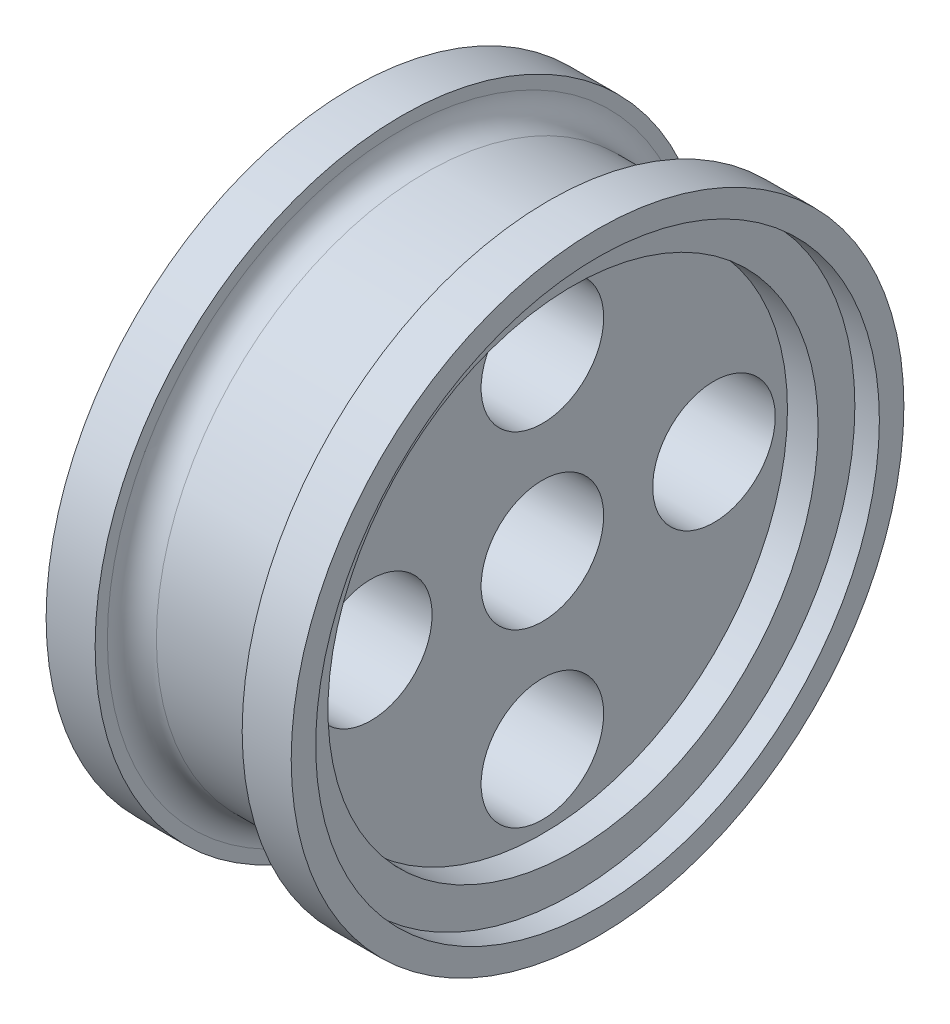
from build123d import *

# Parameters (mm, degrees)
SKETCH2_R          = 11.5
CUT_EXTRUDE1_DEPTH = 1
SKETCH3_R          = 10
CUT_EXTRUDE2_DEPTH = 1.25
SKETCH4_R          = 2.5
CUT_EXTRUDE3_DEPTH = 8.5


with BuildPart() as part:
    # Sketch1 → Revolve1 (revolve)
    with BuildSketch(Plane.XY, mode=Mode.PRIVATE) as revolve1_sk:
        with BuildLine():
            Line((0, 0), (5, 0))
            Line((5, 0), (5, 12.5))
            Line((5, 12.5), (3, 12.5))
            Line((3, 12.5), (3, 12))
            ThreePointArc((3, 12), (2.707106781, 11.292893219), (2, 11))
            Line((2, 11), (0, 11))
            Line((0, 11), (0, 0))
        make_face()
    revolve1 = revolve(revolve1_sk.sketch.rotate(Axis((0, 0, 0), (1, 0, 0)), 90), axis=Axis((0, 0, 0), (1, 0, 0)))

    # Mirror1: Revolve1 across plane
    add(revolve1.mirror(Plane(origin=(0, 0, 0), x_dir=(0, 0, 1), z_dir=(1, 0, 0))))

    # Sketch2 → Cut-Extrude1 (cut)
    with BuildSketch(Plane(origin=(5, 0, 0), x_dir=(0, 0, -1), z_dir=(1, 0, 0))):
        Circle(SKETCH2_R)
    cut_extrude1 = extrude(amount=-CUT_EXTRUDE1_DEPTH, mode=Mode.SUBTRACT)

    # Sketch3 → Cut-Extrude2 (cut)
    with BuildSketch(Plane(origin=(4, 0, 0), x_dir=(0, 0, -1), z_dir=(1, 0, 0))):
        Circle(SKETCH3_R)
    cut_extrude2 = extrude(amount=-CUT_EXTRUDE2_DEPTH, mode=Mode.SUBTRACT)

    # Mirror3: Cut-Extrude1, Cut-Extrude2 across plane
    add(cut_extrude1.mirror(Plane(origin=(0, 0, 0), x_dir=(0, 0, 1), z_dir=(1, 0, 0))), mode=Mode.SUBTRACT)
    add(cut_extrude2.mirror(Plane(origin=(0, 0, 0), x_dir=(0, 0, 1), z_dir=(1, 0, 0))), mode=Mode.SUBTRACT)

    # Sketch4 → Cut-Extrude3 (cut)
    with BuildSketch(Plane(origin=(2.75, 0, 0), x_dir=(0, 0, -1), z_dir=(1, 0, 0))):
        with Locations((0, 7)):
            Circle(SKETCH4_R)
        with Locations((7, 0)):
            Circle(SKETCH4_R)
        with Locations((0, -7)):
            Circle(SKETCH4_R)
        with Locations((-7, 0)):
            Circle(SKETCH4_R)
        Circle(SKETCH4_R)
    extrude(amount=-CUT_EXTRUDE3_DEPTH, mode=Mode.SUBTRACT)


solid = part.part
